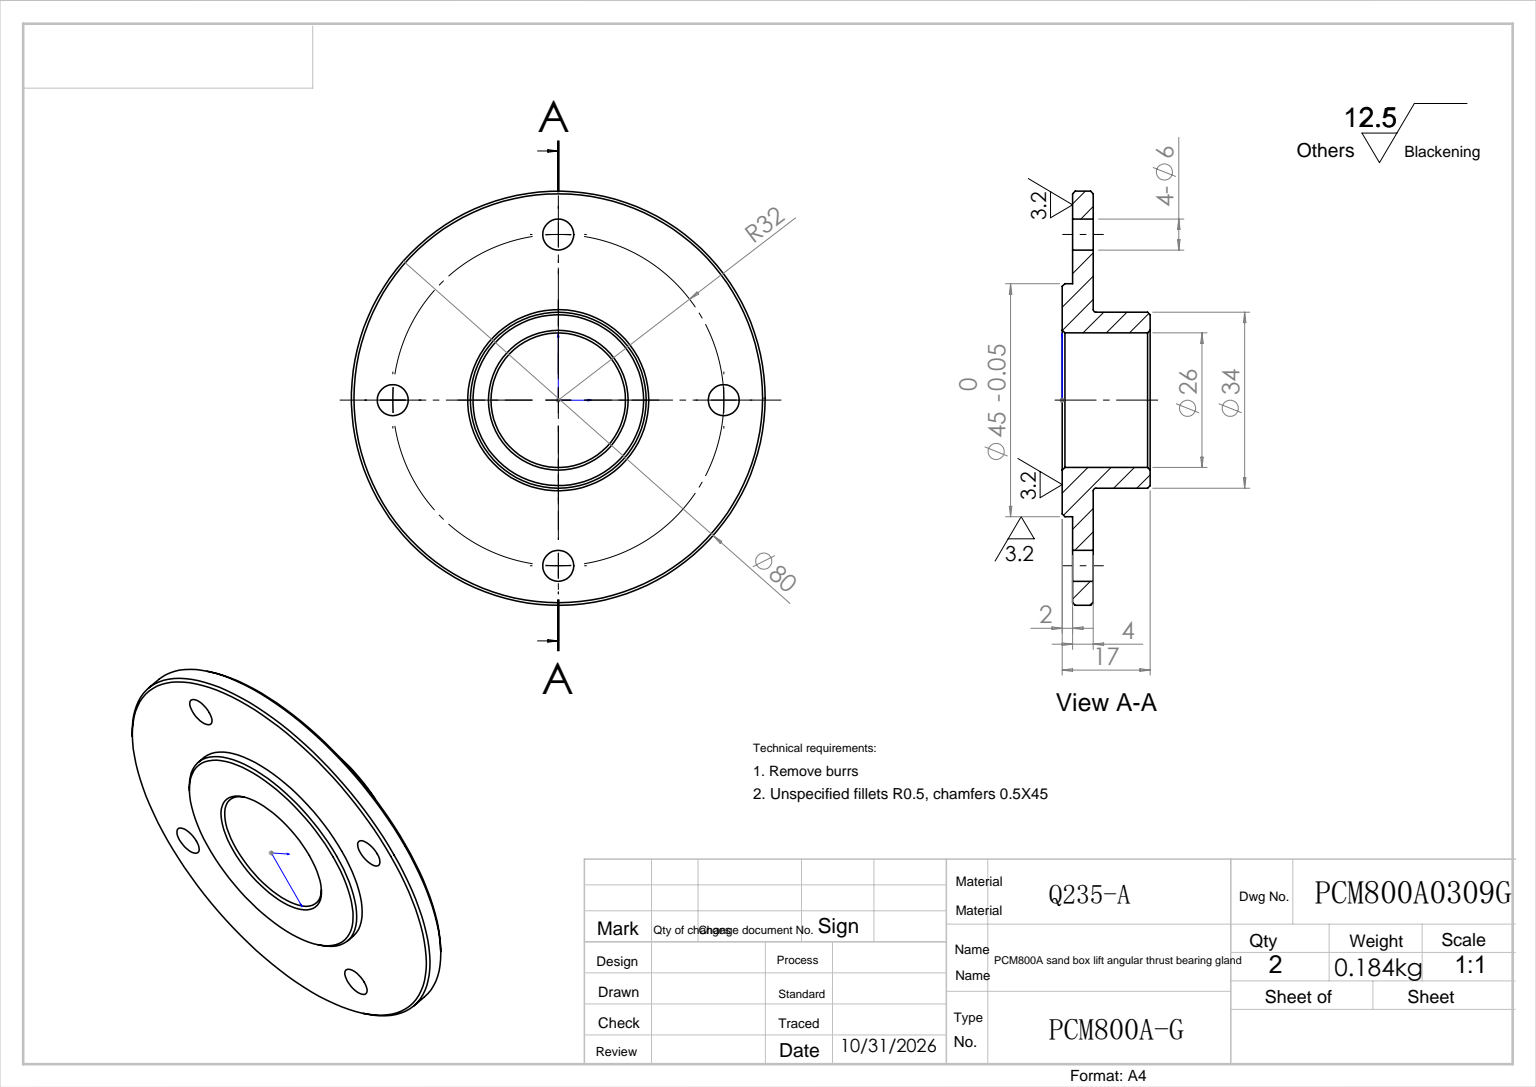
SolidWorks part; units mm, degrees
ref_plane "前视基准面" through (0, 0, 0) normal (0, 0, 1) x (1, 0, 0)
ref_plane "上视基准面" through (0, 0, 0) normal (0, 1, 0) x (1, 0, 0)
ref_plane "右视基准面" through (0, 0, 0) normal (1, 0, 0) x (0, 0, -1)
sketch "草图1" plane through (0, 0, 0) normal (0, 0, 1) x (1, 0, 0)
  circle A0 centre (0, 0) radius 22.5
  circle A1 centre (0, 0) radius 13
extrude "拉伸1" add sketch "草图1" along normal blind 2
sketch "草图2" plane through (0, 0, 2) normal (0, 0, 1) x (1, 0, 0)
  circle A1 centre (0, 0) radius 13
  circle A2 centre (0, 0.3744) radius 40
extrude "拉伸2" add sketch "草图2" along normal blind 4
sketch "草图3" plane through (0, 0, 6) normal (0, 0, 1) x (1, 0, 0)
  circle A0 centre (0, 0) radius 13
  circle A1 centre (0, 0) radius 17
extrude "拉伸3" add sketch "草图3" along normal blind 11
chamfer "倒角1" distance 0.5 angle 45 6 edges at (40, 0.3744, 2) (13, 0, 17) (13, 0, 0) (22.5, 0, 0) (40, 0.3744, 6) (17, 0, 17)
fillet "圆角1" radius 0.5 1 edges at (17, 0, 6)
sketch "草图4" plane through (0, 0, 6) normal (0, 0, 1) x (1, 0, 0)
  circle A0 centre (0, 0) radius 32 construction
  circle A1 centre (0, 32) radius 3
  circle A2 centre (-32, 0) radius 3
  circle A3 centre (0, -32) radius 3
  circle A4 centre (32, 0) radius 3
extrude "切除-拉伸1" cut sketch "草图4" against normal through all
